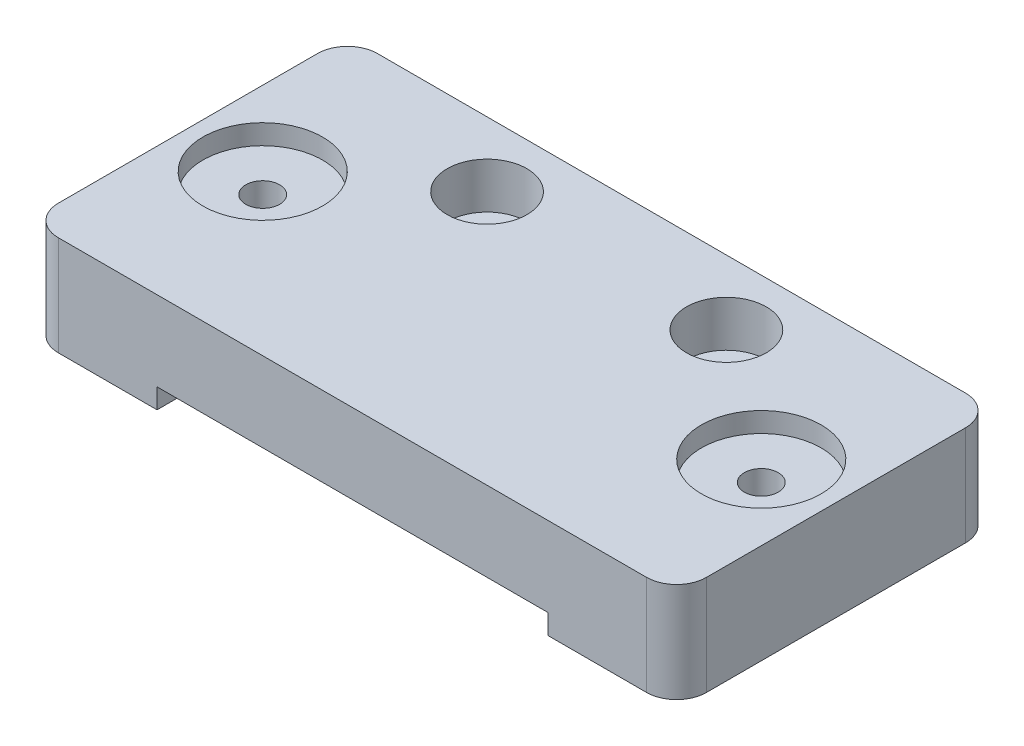
from build123d import *

# Parameters (mm, degrees)
SKETCH_1_W                = 65
SKETCH_1_H                = 10
EXTRUDE_1_DEPTH           = 32
HOLE_WIZARD_5_0_5_1_D     = 4.3
FILLET_1_R                = 3
SKETCH_10_R               = 6
CUT_EXTRUDE_3_DEPTH       = 2
HOLE_WIZARD_1_D           = 3.4
HOLE_WIZARD_1_CBORE_D     = 6
HOLE_WIZARD_1_CBORE_DEPTH = 3.4
HOLE_WIZARD_2_D           = 4.3
HOLE_WIZARD_2_CBORE_D     = 8
HOLE_WIZARD_2_CBORE_DEPTH = 4.6
SKETCH_16_W               = 39.2
SKETCH_16_H               = 72.88385863
CUT_EXTRUDE_4_DEPTH       = 2


with BuildPart() as part:
    # 草图1 → 凸台-拉伸1 (new body)
    with BuildSketch(Plane.XY):
        Rectangle(SKETCH_1_W, SKETCH_1_H)
    extrude(amount=EXTRUDE_1_DEPTH)

    # Ø5.0 (5) 直径孔1 (through all)
    with Locations(Plane.XZ.offset(5)):
        with Locations((-12, 6.5), (12, 6.5)):
            Hole(HOLE_WIZARD_5_0_5_1_D / 2)

    # 圆角1
    fillet_1_edges = [part.edges().sort_by_distance(p)[0] for p in [
        (-32.5, 0, 32),
        (32.5, 0, 32),
        (-32.5, 0, 0),
        (32.5, 0, 0),
    ]]
    fillet(fillet_1_edges, radius=FILLET_1_R)

    # 草图10 → 切除-拉伸3 (cut)
    with BuildSketch(Plane(origin=(0, 5, 0), x_dir=(1, 0, 0), z_dir=(0, 1, 0))):
        with Locations(Location((-25, -16, 0), (0, 0, 270))):
            Circle(SKETCH_10_R)
        with Locations(Location((25, -16, 0), (0, 0, 90))):
            Circle(SKETCH_10_R)
    extrude(amount=-CUT_EXTRUDE_3_DEPTH, mode=Mode.SUBTRACT)

    # 打孔尺寸(%根据)开槽圆柱头螺钉的类型1 (through all)
    with Locations(Plane(origin=(0, -5, 0), x_dir=(-1, 0, 0), z_dir=(0, -1, 0))):
        with Locations((-25, -16), (25, -16)):
            CounterBoreHole(HOLE_WIZARD_1_D / 2, HOLE_WIZARD_1_CBORE_D / 2, HOLE_WIZARD_1_CBORE_DEPTH)

    # 打孔尺寸(%根据)开槽圆柱头螺钉的类型2 (through all)
    with Locations(Plane(origin=(0, 5, 0), x_dir=(1, 0, 0), z_dir=(0, 1, 0))):
        with Locations((-12, -6.5), (12, -6.5)):
            CounterBoreHole(HOLE_WIZARD_2_D / 2, HOLE_WIZARD_2_CBORE_D / 2, HOLE_WIZARD_2_CBORE_DEPTH)

    # 草图16 → 切除-拉伸4 (cut)
    with BuildSketch(Plane.XZ.offset(5)):
        Rectangle(SKETCH_16_W, SKETCH_16_H)
    extrude(amount=-CUT_EXTRUDE_4_DEPTH, mode=Mode.SUBTRACT)


solid = part.part
